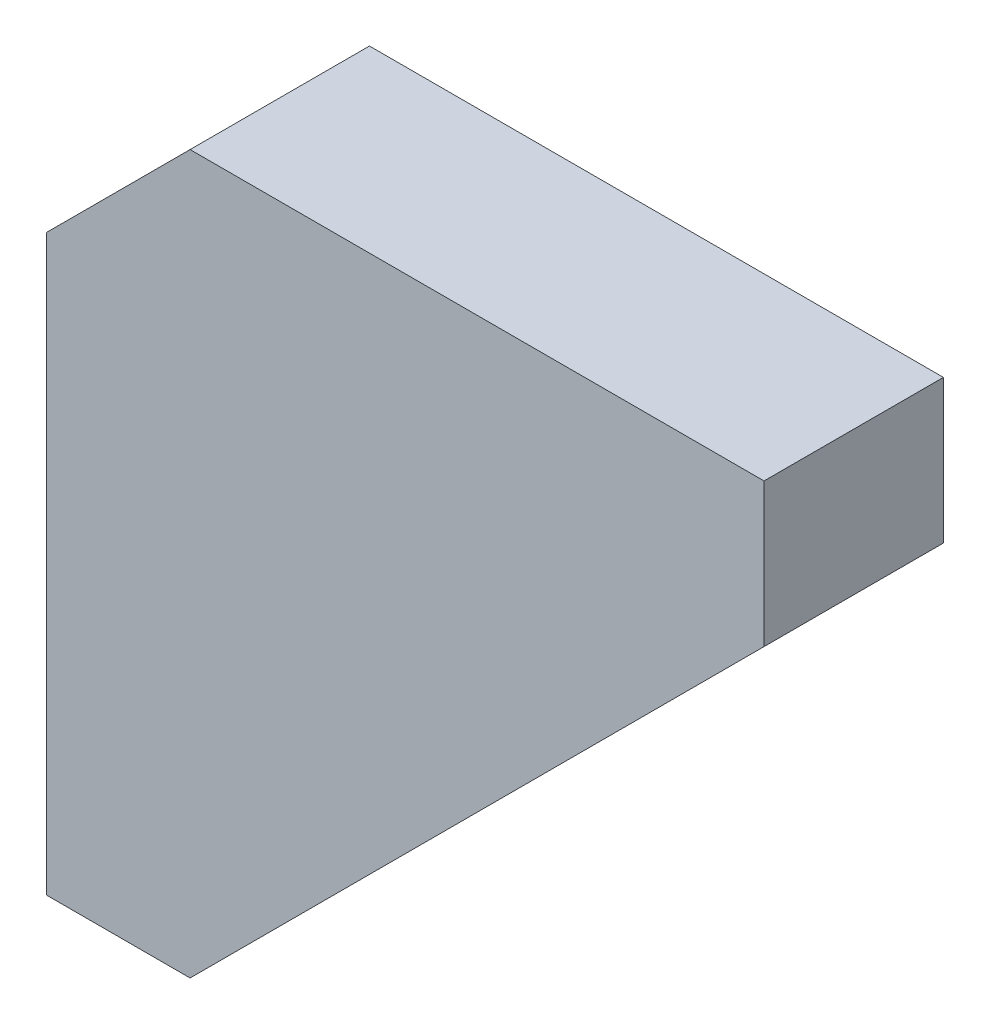
SolidWorks part; units mm, degrees
material "普通碳钢"
ref_plane "Front Plane" through (0, 0, 0) normal (0, 0, 1) x (1, 0, 0)
ref_plane "Top Plane" through (0, 0, 0) normal (0, 1, 0) x (1, 0, 0)
ref_plane "Right Plane" through (0, 0, 0) normal (1, 0, 0) x (0, 0, -1)
sketch "Sketch1" plane through (0, 0, 0) normal (0, 0, 1) x (1, 0, 0)
  line L0 (0, 0) -> (20, 0)
  line L1 (20, 0) -> (100, 80)
  line L2 (100, 80) -> (100, 100)
  line L3 (100, 100) -> (20, 100)
  line L4 (0, 80) -> (0, 0)
  line L5 (20, 100) -> (0, 80)
  point P6 (0, 100)
  dimension "D1" = 100
  dimension "D2" = 100
  dimension "D3" = 20
  dimension "D4" = 20
extrude "Boss-Extrude1" add sketch "Sketch1" along normal blind 25
